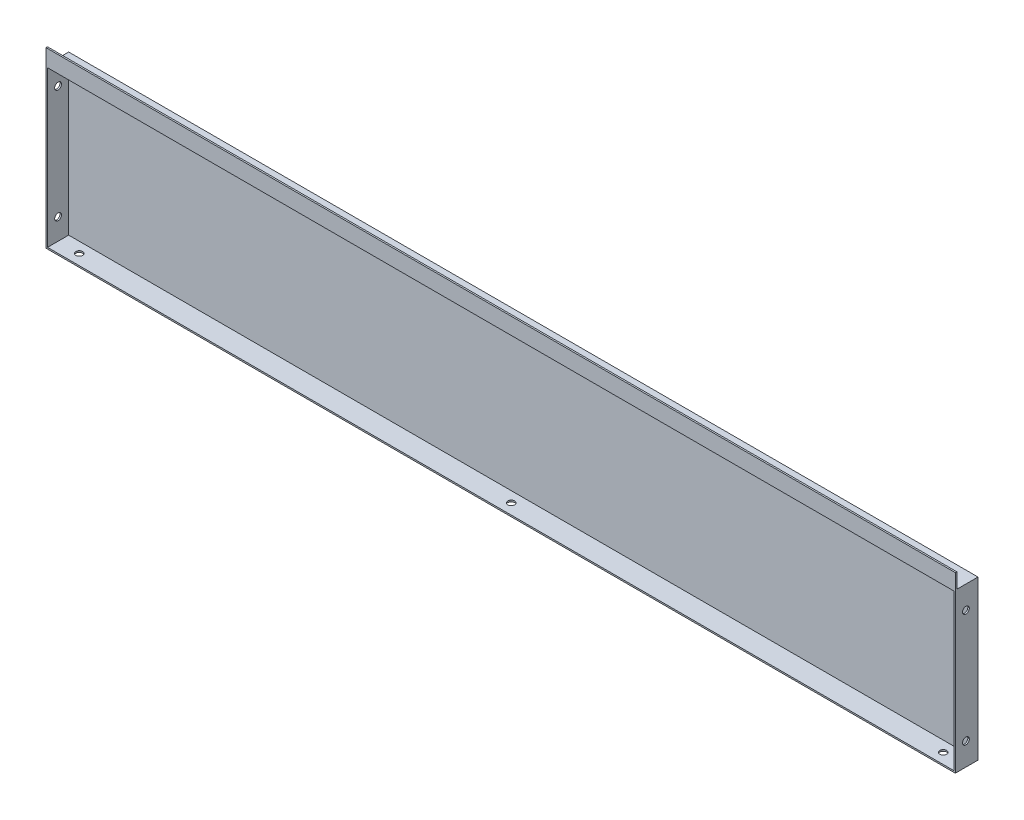
SolidWorks part; units mm, degrees
ref_plane "前视基准面" through (0, 0, 0) normal (0, 0, 1) x (1, 0, 0)
ref_plane "上视基准面" through (0, 0, 0) normal (0, 1, 0) x (1, 0, 0)
ref_plane "右视基准面" through (0, 0, 0) normal (1, 0, 0) x (0, 0, -1)
sketch "草图1" plane through (0, 0, 0) normal (0, 0, 1) x (1, 0, 0)
  line L1 (0, 0) -> (1204, 0)
  line L2 (0, 0) -> (0, 210)
  line L3 (0, 210) -> (1204, 210)
  line L4 (1204, 0) -> (1204, 210)
  dimension "D1" = 210
  dimension "D2" = 1204
extrude "凸台-拉伸1" add sketch "草图1" along normal blind 30
shell "抽壳1" thickness 2
sketch "草图2" plane through (0, 0, 30) normal (0, 0, 1) x (1, 0, 0)
  line L0 (1202, 208) -> (2, 208) construction
  line L1 (0, 230) -> (1204, 230)
  line L2 (0, 230) -> (0, 210)
  line L3 (0, 210) -> (1204, 210)
  line L4 (1204, 210) -> (1204, 230)
  line L6 (1204, 210) -> (0, 210) construction
  dimension "D1" = 20
extrude "凸台-拉伸2" add sketch "草图2" against normal blind 2
sketch "草图3" plane through (2, 0, 0) normal (1, 0, 0) x (0, 0, -1)
  line L0 (-16, 2) -> (-16, 272.4876) construction
  line L1 (-30, 2) -> (-2, 2) construction
  line L2 (-30, 0) -> (0, 0) construction
  line L3 (-28, 210) -> (0, 210) construction
  circle A0 centre (-16, 180) radius 4.5
  circle A1 centre (-16, 30) radius 4.5
  dimension "D1" = 9
  dimension "D2" = 9
  dimension "D3" = 30
  dimension "D4" = 30
extrude "切除-拉伸1" cut sketch "草图3" against normal blind 116 and the other way blind 1477
sketch "草图4" plane through (0, 2, 0) normal (0, 1, 0) x (1, 0, 0)
  line L0 (2, -16) -> (1260.3911, -16) construction
  line L1 (2, -30) -> (2, -2) construction
  line L2 (602, -28) -> (602, 174.5599) construction
  line L3 (0, -28) -> (1204, -28) construction
  line L4 (0, -30) -> (0, 0) construction
  line L5 (1204, -30) -> (1204, 0) construction
  circle A0 centre (30, -16) radius 4.5
  circle A1 centre (1174, -16) radius 4.5
  circle A2 centre (602, -16) radius 4.5
  dimension "D1" = 9
  dimension "D2" = 9
  dimension "D3" = 9
  dimension "D4" = 30
  dimension "D5" = 30
extrude "切除-拉伸2" cut sketch "草图4" against normal blind 116
